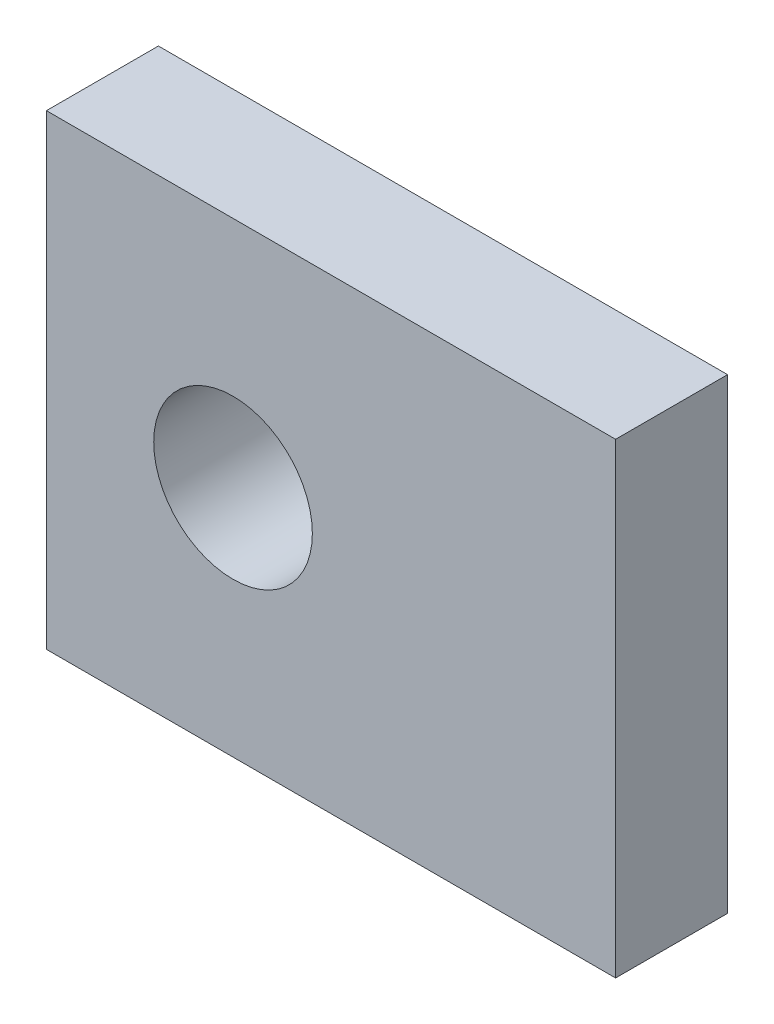
SolidWorks part; units mm, degrees
ref_plane "Front Plane" through (0, 0, 0) normal (0, 0, 1) x (1, 0, 0)
ref_plane "Top Plane" through (0, 0, 0) normal (0, 1, 0) x (1, 0, 0)
ref_plane "Right Plane" through (0, 0, 0) normal (1, 0, 0) x (0, 0, -1)
sketch "Sketch1" plane through (0, 0, 0) normal (0, 0, 1) x (1, 0, 0)
  line L1 (-36.6, -43.1057) -> (-6.1, -43.1057)
  line L2 (-36.6, -43.1057) -> (-36.6, -68.1057)
  line L3 (-36.6, -68.1057) -> (-6.1, -68.1057)
  line L4 (-6.1, -43.1057) -> (-6.1, -68.1057)
  circle A0 centre (-26.6, -55.6057) radius 4.25
extrude "Boss-Extrude1" add sketch "Sketch1" along normal blind 6
